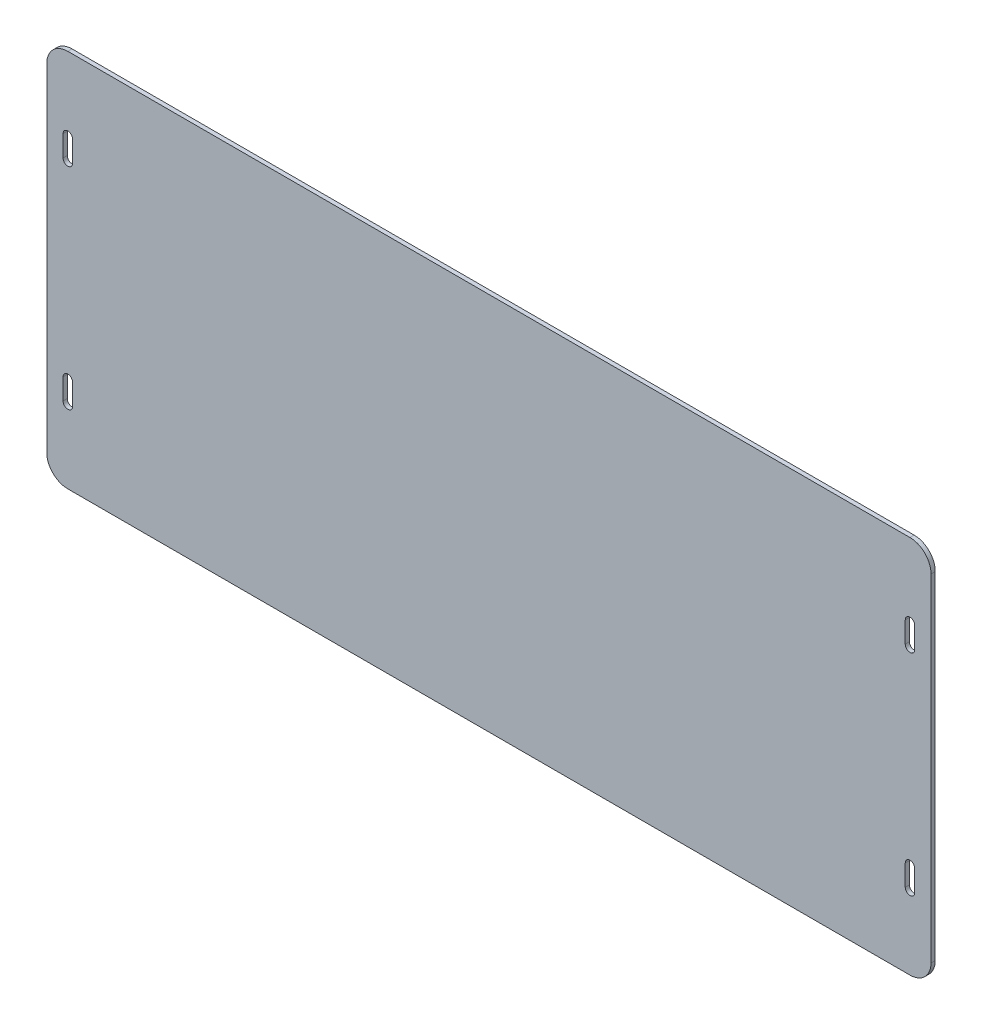
from build123d import *

# Parameters (mm, degrees)
SKETCH_1_W          = 420
SKETCH_1_H          = 180
EXTRUDE_1_DEPTH     = 2
HOLE_WIZARD_M4_2_D  = 3.3
CUT_EXTRUDE_1_DEPTH = 10
FILLET_1_R          = 10


with BuildPart() as part:
    # 草图1 → 凸台-拉伸1 (new body)
    with BuildSketch(Plane.XY):
        Rectangle(SKETCH_1_W, SKETCH_1_H)
    extrude(amount=EXTRUDE_1_DEPTH)

    # M4 螺纹孔的螺纹孔钻头2 (through all)
    with Locations(Plane.XY.offset(2)):
        with Locations((200, 50), (-200, -50), (-200, 50), (200, -50)):
            Hole(HOLE_WIZARD_M4_2_D / 2)

    # 草图4 → 切除-拉伸1 (cut)
    with BuildSketch(Plane.XY.offset(2)):
        with BuildLine():
            Line((202.25, 55), (202.25, 45))
            ThreePointArc((202.25, 45), (200, 42.75), (197.75, 45))
            Line((197.75, 45), (197.75, 55))
            ThreePointArc((197.75, 55), (200, 57.25), (202.25, 55))
        make_face()
        with BuildLine():
            Line((197.75, -55), (197.75, -45))
            ThreePointArc((197.75, -45), (200, -42.75), (202.25, -45))
            Line((202.25, -45), (202.25, -55))
            ThreePointArc((202.25, -55), (200, -57.25), (197.75, -55))
        make_face()
        with BuildLine():
            Line((-197.75, -55), (-197.75, -45))
            ThreePointArc((-197.75, -45), (-200, -42.75), (-202.25, -45))
            Line((-202.25, -45), (-202.25, -55))
            ThreePointArc((-202.25, -55), (-200, -57.25), (-197.75, -55))
        make_face()
        with BuildLine():
            Line((-202.25, 55), (-202.25, 45))
            ThreePointArc((-202.25, 45), (-200, 42.75), (-197.75, 45))
            Line((-197.75, 45), (-197.75, 55))
            ThreePointArc((-197.75, 55), (-200, 57.25), (-202.25, 55))
        make_face()
    extrude(amount=-CUT_EXTRUDE_1_DEPTH, mode=Mode.SUBTRACT)

    # 圆角1
    fillet_1_edges = [part.edges().sort_by_distance(p)[0] for p in [
        (210, -90, 1),
        (-210, -90, 1),
        (-210, 90, 1),
        (210, 90, 1),
    ]]
    fillet(fillet_1_edges, radius=FILLET_1_R)


solid = part.part
